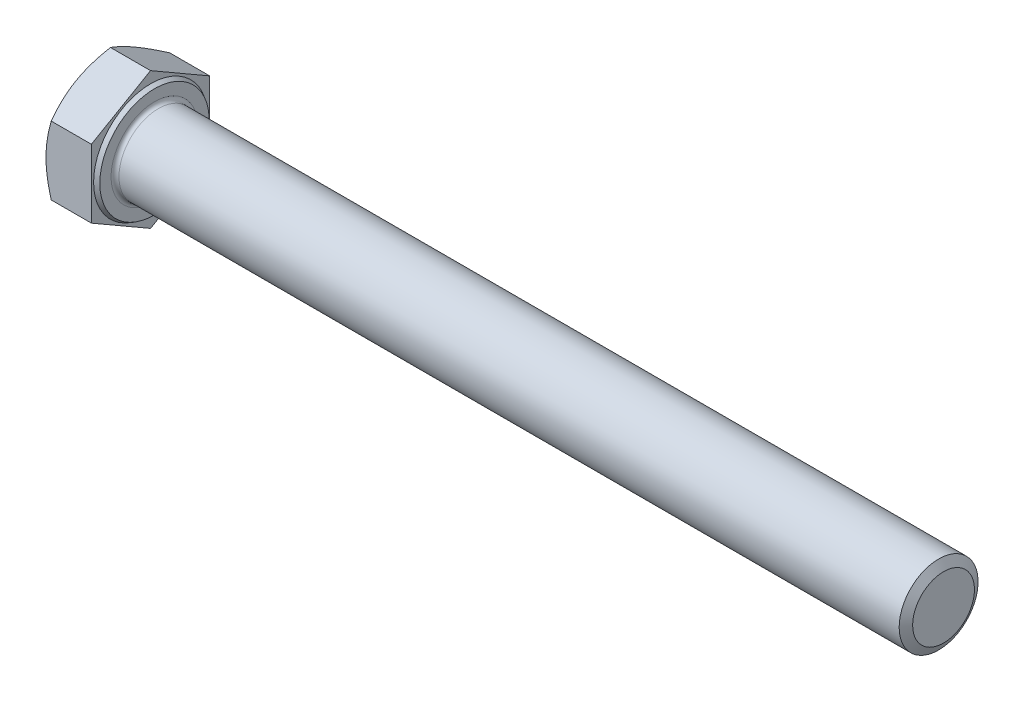
from build123d import *

# Parameters (mm, degrees)
EXTRUDE_421_DEPTH = 7.5
FILLET_1347_R     = 0.6


with BuildPart() as part:
    # 草图1 → Extrude 421 (new body)
    with BuildSketch(Plane(origin=(0, 0, 0), x_dir=(0, 0, -1), z_dir=(1, 0, 0))):
        Polygon((9, 5.196152423), (9, -5.196152423), (0, -10.392304845), (-9, -5.196152423), (-9, 5.196152423), (0, 10.392304845), align=None)
    extrude(amount=EXTRUDE_421_DEPTH)

    # 草图2 → 凸台-旋转1 (revolve)
    with BuildSketch(Plane.XY, mode=Mode.PRIVATE) as revolve_1_sk:
        Polygon((0, 0), (127.5, 0), (127.5, 4.701), (127.5, 6), (63.75, 6), (0, 6), align=None)
    revolve(revolve_1_sk.sketch.rotate(Axis((0, 0, 0), (1, 0, 0)), 90), axis=Axis((0, 0, 0), (1, 0, 0)))

    # 草图3 → 切除-旋转1 (revolve, cut)
    with BuildSketch(Plane.XY):
        Polygon((0, 9), (3.690598923, 15.392304845), (3.690598923, 20.392304845), (-10, 20.392304845), (-10, 9), align=None)
    revolve(axis=Axis((0, 0, 0), (1, 0, 0)), mode=Mode.SUBTRACT)

    # 草图4 → 切除-旋转3 (revolve, cut)
    with BuildSketch(Plane.XY, mode=Mode.PRIVATE) as cut_revolve_3_sk:
        Polygon((7.5, 8.315), (6.9, 8.661410162), (6.9, 10.392304845), (7.5, 10.392304845), align=None)
    revolve(cut_revolve_3_sk.sketch.rotate(Axis((0, 0, 0), (1, 0, 0)), 90), axis=Axis((0, 0, 0), (1, 0, 0)), mode=Mode.SUBTRACT)

    # Fillet 1347
    fillet_1347_edges = [part.edges().sort_by_distance(p)[0] for p in [
        (7.5, 0, -6),
    ]]
    fillet(fillet_1347_edges, radius=FILLET_1347_R)

    # 草图6 → 切除-旋转4 (revolve, cut)
    with BuildSketch(Plane.XY, mode=Mode.PRIVATE) as cut_revolve_4_sk:
        Polygon((126.75, 6), (128.25, 6), (127.5, 4.700961894), align=None)
    revolve(cut_revolve_4_sk.sketch.rotate(Axis((0, 0, 0), (1, 0, 0)), 90), axis=Axis((0, 0, 0), (1, 0, 0)), mode=Mode.SUBTRACT)


solid = part.part
